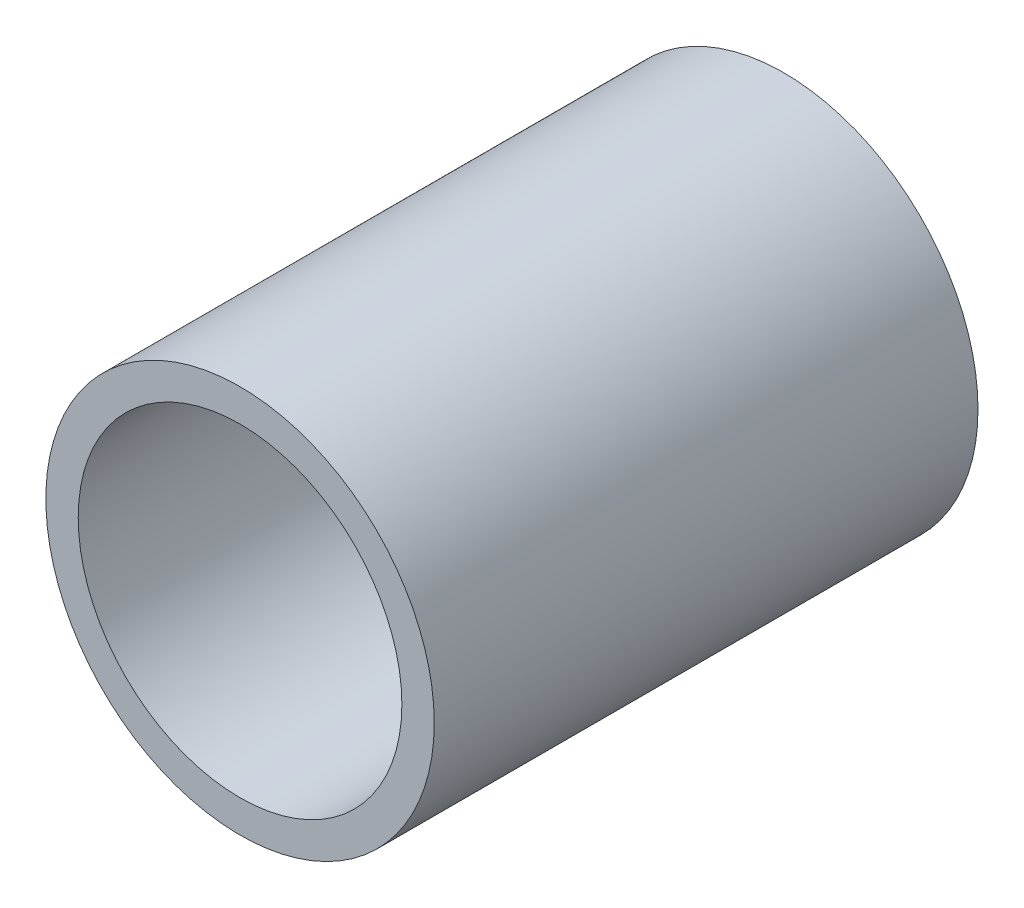
SolidWorks part; units mm, degrees
ref_plane "Front Plane" through (0, 0, 0) normal (0, 0, 1) x (1, 0, 0)
ref_plane "Top Plane" through (0, 0, 0) normal (0, 1, 0) x (1, 0, 0)
ref_plane "Right Plane" through (0, 0, 0) normal (1, 0, 0) x (0, 0, -1)
sketch "Sketch1" plane through (0, 0, 0) normal (0, 0, 1) x (1, 0, 0)
  circle A0 centre (0, 0) radius 5
  circle A1 centre (0, 0) radius 6
  dimension "D1" = 10
  dimension "D2" = 12
extrude "Boss-Extrude1" add sketch "Sketch1" along normal mid plane 16.8
